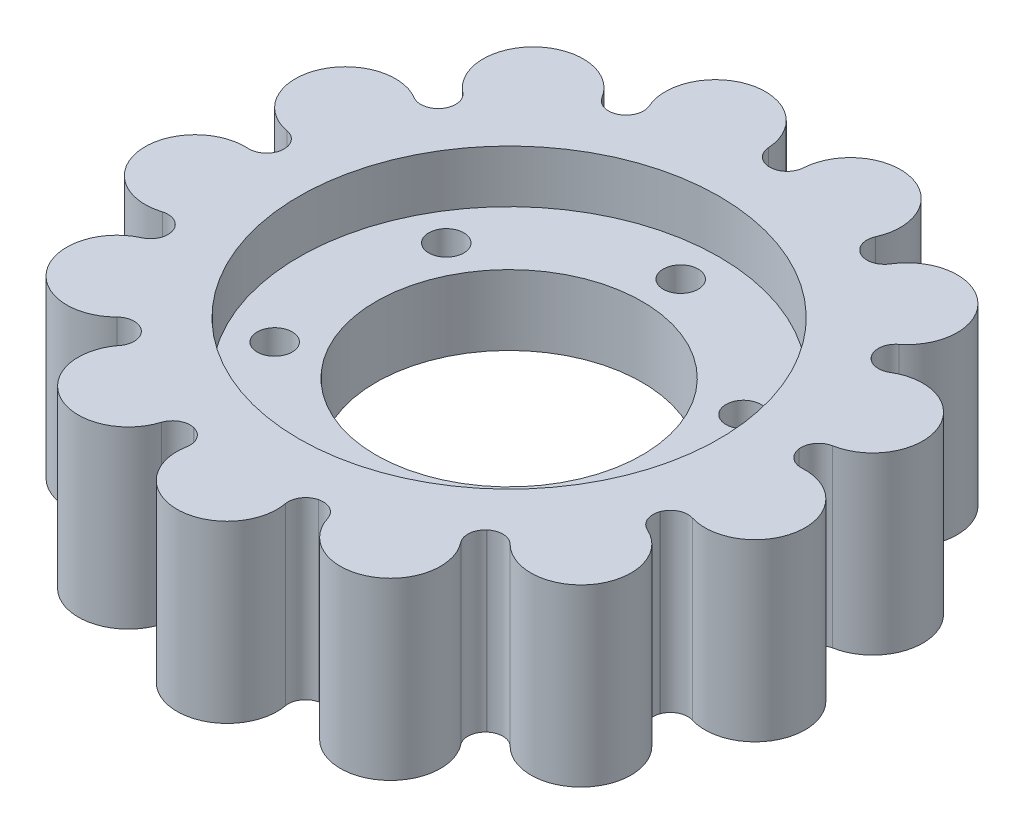
from build123d import *

# Parameters (mm, degrees)
EXTRUDE_1_DEPTH          = 25
SKETCH_3_R               = 74.389991886
SKETCH_3_R_2             = 60
EXTRUDE_2_DEPTH          = 25
PATTERN_CIRCULAR_1_COUNT = 13
SKETCH_4_R               = 60
SKETCH_4_R_2             = 38
SKETCH_4_R_3             = 5
EXTRUDE_3_DEPTH          = 10


with BuildPart() as part:
    # 草图2 → 凸台-拉伸1 (new, symmetric)
    with BuildSketch(Plane(origin=(0, 0, 0), x_dir=(1, 0, 0), z_dir=(0, 1, 0))):
        with BuildLine():
            ThreePointArc((-34.536040721, 65.887273309), (-17.783660561, 72.233041676), (0, 74.389991886))
            ThreePointArc((0, 74.389991886), (-3.422380364, 75.744820223), (-4.990060614, 79.075079343))
            ThreePointArc((-4.990060614, 79.075079343), (-4.990234092, 79.075068396), (-4.990407571, 79.075057448))
            ThreePointArc((-4.990407571, 79.075057448), (-22.715686348, 92.058757055), (-32.30963725, 72.292167331))
            ThreePointArc((-32.30963725, 72.292167331), (-32.171226647, 68.654647695), (-34.536040721, 65.887273309))
        make_face()
    extrude_1 = extrude(amount=EXTRUDE_1_DEPTH, both=True)

    # 草图3 → 凸台-拉伸2 (add, symmetric)
    with BuildSketch(Plane(origin=(0, 0, 0), x_dir=(1, 0, 0), z_dir=(0, 1, 0))):
        Circle(SKETCH_3_R)
        with Locations(Location((0, 0, 0), (0, 0, 270))):
            Circle(SKETCH_3_R_2, mode=Mode.SUBTRACT)
    extrude(amount=EXTRUDE_2_DEPTH, both=True)

    # 阵列(圆周)1: 凸台-拉伸1 ×13 about axis
    pattern_circular_1_axis = Axis((0, 0, 0), (0, 1, 0))
    for i in range(1, PATTERN_CIRCULAR_1_COUNT):
        add(extrude_1.rotate(pattern_circular_1_axis, i * 360 / PATTERN_CIRCULAR_1_COUNT))

    # 草图4 → 凸台-拉伸3 (add, symmetric)
    with BuildSketch(Plane(origin=(0, 0, 0), x_dir=(1, 0, 0), z_dir=(0, 1, 0))):
        with Locations(Location((0, 0, 0), (0, 0, 270))):
            Circle(SKETCH_4_R)
        with Locations(Location((0, 0, 0), (0, 0, 270))):
            Circle(SKETCH_4_R_2, mode=Mode.SUBTRACT)
        with Locations(Location((0, 49, 0), (0, 0, 270))):
            Circle(SKETCH_4_R_3, mode=Mode.SUBTRACT)
        with Locations(Location((42.435244785, 24.5, 0), (0, 0, 270))):
            Circle(SKETCH_4_R_3, mode=Mode.SUBTRACT)
        with Locations(Location((42.435244785, -24.5, 0), (0, 0, 270))):
            Circle(SKETCH_4_R_3, mode=Mode.SUBTRACT)
        with Locations(Location((0, -49, 0), (0, 0, 270))):
            Circle(SKETCH_4_R_3, mode=Mode.SUBTRACT)
        with Locations(Location((-42.435244785, -24.5, 0), (0, 0, 270))):
            Circle(SKETCH_4_R_3, mode=Mode.SUBTRACT)
        with Locations(Location((-42.435244785, 24.5, 0), (0, 0, 270))):
            Circle(SKETCH_4_R_3, mode=Mode.SUBTRACT)
    extrude(amount=EXTRUDE_3_DEPTH, both=True)


solid = part.part
